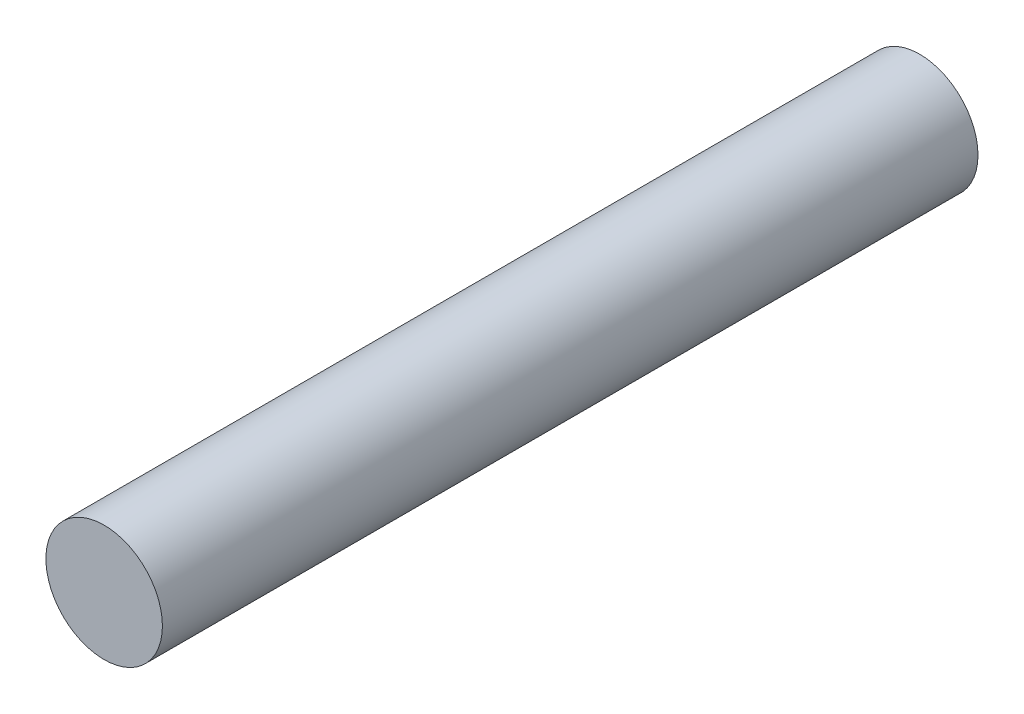
from build123d import *

# Parameters (mm, degrees)
BOSS_EXTRUDE1_DEPTH      = 250
BOSS_EXTRUDE1_DEPTH_BACK = 30
SKETCH1_R                = 20


with BuildPart() as part:
    # Sketch1 → Boss-Extrude1 (new, two sides: drawn at the far end of the back side and taken through both)
    with BuildSketch(Plane.XY.offset(-BOSS_EXTRUDE1_DEPTH_BACK)):
        Circle(SKETCH1_R)
    extrude(amount=BOSS_EXTRUDE1_DEPTH + BOSS_EXTRUDE1_DEPTH_BACK)


solid = part.part
